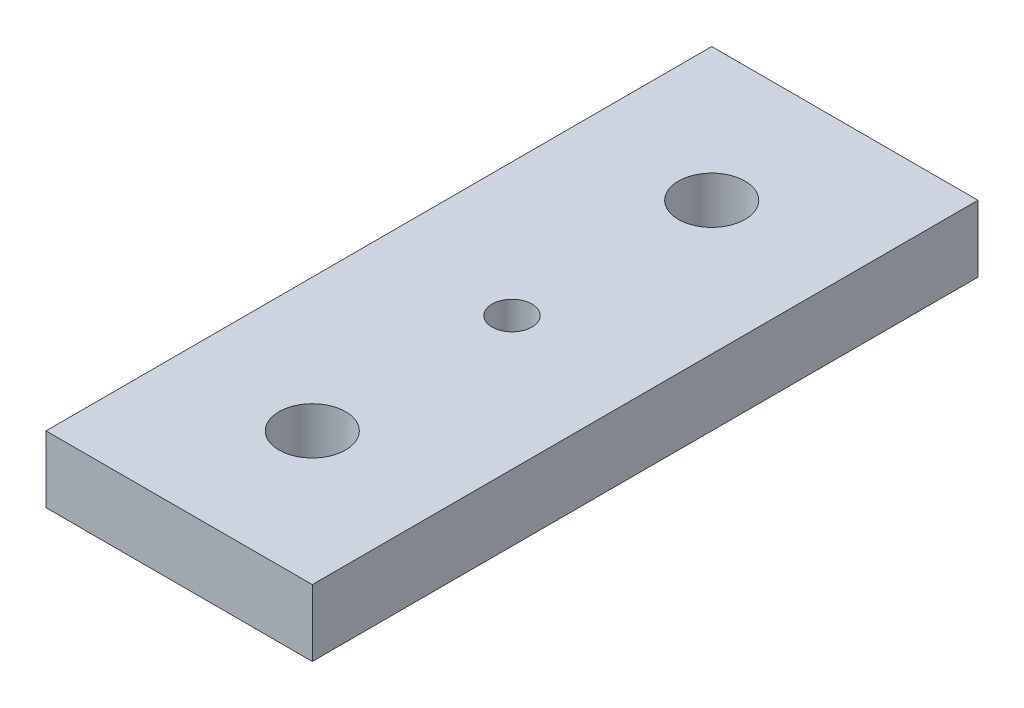
from build123d import *

# Parameters (mm, degrees)
SKETCH1_W           = 40
SKETCH1_H           = 100
SKETCH1_R           = 5
SKETCH1_R_2         = 3
BOSS_EXTRUDE1_DEPTH = 10


with BuildPart() as part:
    # Sketch1 → Boss-Extrude1 (new body)
    with BuildSketch(Plane(origin=(0, 0, 0), x_dir=(1, 0, 0), z_dir=(0, 1, 0))):
        Rectangle(SKETCH1_W, SKETCH1_H)
        with Locations(Location((0, 30, 0), (0, 0, 270))):
            Circle(SKETCH1_R, mode=Mode.SUBTRACT)
        with Locations(Location((0, -30, 0), (0, 0, 270))):
            Circle(SKETCH1_R, mode=Mode.SUBTRACT)
        with Locations(Location((0, 0, 0), (0, 0, 270))):
            Circle(SKETCH1_R_2, mode=Mode.SUBTRACT)
    extrude(amount=BOSS_EXTRUDE1_DEPTH)


solid = part.part
